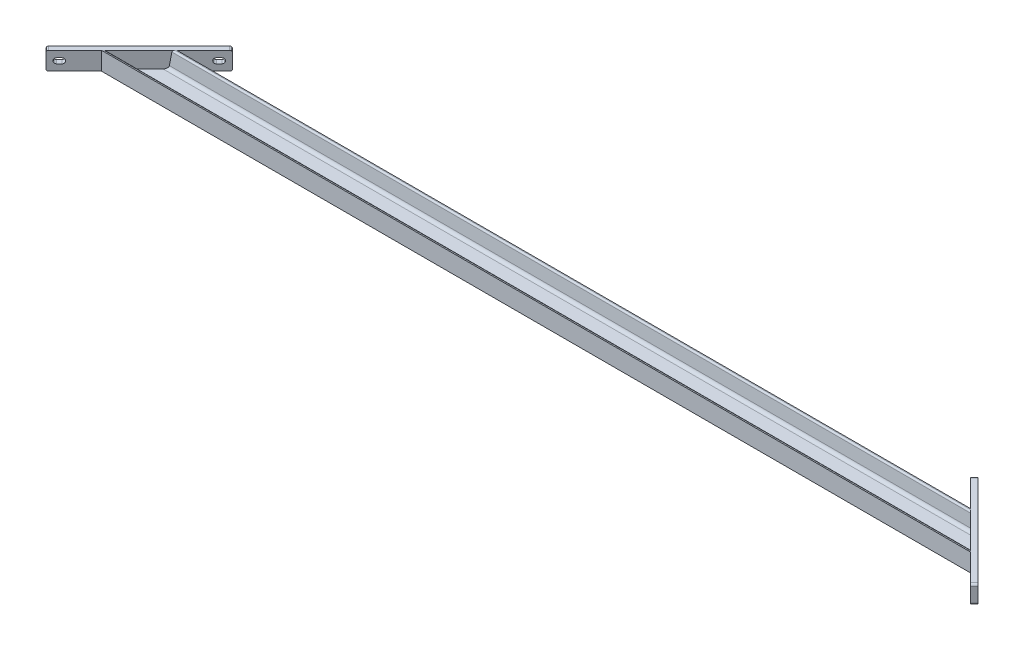
from build123d import *

# Parameters (mm, degrees)
GB_T707_1988_HOT_ROLLED_CHANNEL_10_1_DEPTH = 2307.5
CUT_EXTRUDE1_DEPTH                         = 1156.830031839
BOSS_EXTRUDE1_DEPTH                        = 14


with BuildPart() as part:
    # Sketch1 → Gb／t707-1988 Hot-Rolled Channel 10(1) (new body)
    with BuildSketch(Plane(origin=(-1153.75, 0, -50), x_dir=(0, 1, 0), z_dir=(1, 0, 0))):
        with BuildLine():
            Line((48, 100), (0, 100))
            Line((0, 100), (0, 0))
            Line((0, 0), (48, 0))
            Line((48, 0), (48, 2.474327591))
            ThreePointArc((48, 2.474327591), (46.921208267, 5.284676138), (44.239019546, 6.651319552))
            Line((44.239019546, 6.651319552), (12.911508062, 9.943973689))
            ThreePointArc((12.911508062, 9.943973689), (7.483268983, 12.709799645), (5.3, 18.397409799))
            Line((5.3, 18.397409799), (5.3, 81.602590201))
            ThreePointArc((5.3, 81.602590201), (7.483268983, 87.290200355), (12.911508062, 90.056026311))
            Line((12.911508062, 90.056026311), (44.239019546, 93.348680448))
            ThreePointArc((44.239019546, 93.348680448), (46.921208267, 94.715323862), (48, 97.525672409))
            Line((48, 97.525672409), (48, 100))
        make_face()
    extrude(amount=GB_T707_1988_HOT_ROLLED_CHANNEL_10_1_DEPTH)

    # Sketch3 → Cut-Extrude1 (cut, through all)
    with BuildSketch(Plane.XZ):
        Polygon((1153.75, 50), (1053.75, -50), (1153.75, -50), align=None)
        Polygon((-1153.75, 50), (-1153.75, -50), (-1053.75, -50), align=None)
    extrude(amount=-CUT_EXTRUDE1_DEPTH, mode=Mode.SUBTRACT)


with BuildPart() as body_2:
    # Sketch4 → Boss-Extrude1 (new body)
    with BuildSketch(Plane(origin=(-551.875, 0, -551.875), x_dir=(-0.7071067811865479, 0, 0.7071067811865472), z_dir=(-0.7071067811865472, 0, -0.7071067811865479))):
        with BuildLine():
            Line((610.469109735, 0), (950.469109735, 0))
            ThreePointArc((950.469109735, 0), (954.004643641, 1.464466094), (955.469109735, 5))
            Line((955.469109735, 5), (955.469109735, 43))
            ThreePointArc((955.469109735, 43), (954.004643641, 46.535533906), (950.469109735, 48))
            Line((950.469109735, 48), (610.469109735, 48))
            ThreePointArc((610.469109735, 48), (606.933575829, 46.535533906), (605.469109735, 43))
            Line((605.469109735, 43), (605.469109735, 5))
            ThreePointArc((605.469109735, 5), (606.933575829, 1.464466094), (610.469109735, 0))
        make_face()
        with BuildLine():
            Line((925.469109735, 31), (935.469109735, 31))
            ThreePointArc((935.469109735, 31), (942.469109735, 24), (935.469109735, 17))
            Line((935.469109735, 17), (925.469109735, 17))
            ThreePointArc((925.469109735, 17), (918.469109735, 24), (925.469109735, 31))
        make_face(mode=Mode.SUBTRACT)
        with BuildLine():
            Line((625.469109735, 31), (635.469109735, 31))
            ThreePointArc((635.469109735, 31), (642.469109735, 24), (635.469109735, 17))
            Line((635.469109735, 17), (625.469109735, 17))
            ThreePointArc((625.469109735, 17), (618.469109735, 24), (625.469109735, 31))
        make_face(mode=Mode.SUBTRACT)
    extrude(amount=BOSS_EXTRUDE1_DEPTH)


with BuildPart() as body_3:
    # Mirror1: mirrored copy
    add(body_2.part.mirror(Plane(origin=(0, 0, 0), x_dir=(0, 0, 1), z_dir=(1, 0, 0))))


solid = Compound([part.part, body_2.part, body_3.part])
